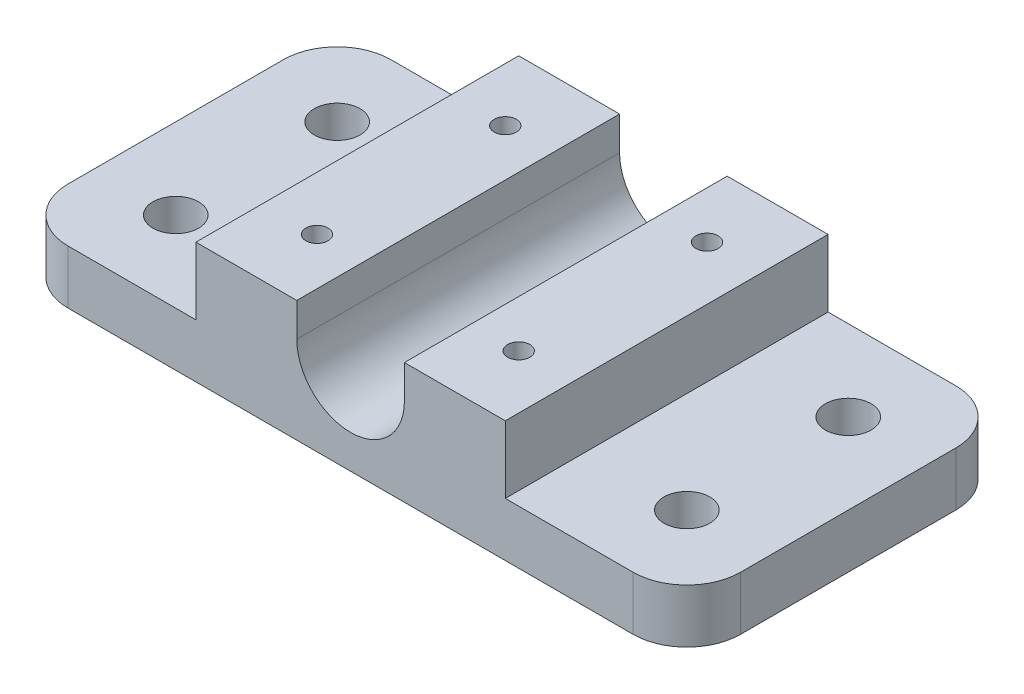
SolidWorks part; units mm, degrees
ref_plane "Front Plane" through (0, 0, 0) normal (0, 0, 1) x (1, 0, 0)
ref_plane "Top Plane" through (0, 0, 0) normal (0, 1, 0) x (1, 0, 0)
ref_plane "Right Plane" through (0, 0, 0) normal (1, 0, 0) x (0, 0, -1)
sketch "Sketch1" plane through (0, 0, 0) normal (0, 1, 0) x (1, 0, 0)
  line L1 (-50, 24) -> (50, 24)
  line L2 (-50, 24) -> (-50, -24)
  line L3 (-50, -24) -> (50, -24)
  line L4 (50, 24) -> (50, -24)
  line L5 (-50, 24) -> (50, -24) construction
  line L6 (-50, -24) -> (50, 24) construction
  point P0 (0, 0)
  dimension "D1" = 100
  dimension "D2" = 48
extrude "Boss-Extrude1" add sketch "Sketch1" along normal blind 8
sketch "Sketch2" plane through (0, 8, 0) normal (0, 1, 0) x (1, 0, 0)
  line L0 (-50, -24) -> (50, -24) construction
  line L1 (-23, 24) -> (23, 24)
  line L2 (-23, 24) -> (-23, -24)
  line L3 (-23, -24) -> (23, -24)
  line L4 (23, 24) -> (23, -24)
  line L5 (-23, 24) -> (23, -24) construction
  line L6 (-23, -24) -> (23, 24) construction
  point P0 (0, 0)
  dimension "D1" = 46
extrude "Boss-Extrude2" add sketch "Sketch2" along normal blind 10
sketch "Sketch3" plane through (0, 0, 24) normal (0, 0, 1) x (1, 0, 0)
  line L0 (0, 21) -> (0, 18) construction
  line L1 (-23, 18) -> (23, 18) construction
  line L3 (0, 13) -> (0, 18) construction
  line L4 (0, 5) -> (0, 18) construction
  line L5 (-8, 13) -> (-8, 18)
  line L6 (8, 13) -> (8, 18)
  line L7 (-8, 18) -> (8, 18)
  arc A0 (-8, 13) -> (8, 13) centre (0, 13) ccw
  dimension "D1" = 16
  dimension "D2" = 3
  dimension "D3" = 5
  dimension "D4" = 13
extrude "Cut-Extrude1" cut sketch "Sketch3" against normal through all
fillet "Fillet1" radius 8 4 edges at (50, 4, -24) (50, 4, 24) (-50, 4, -24) (-50, 4, 24)
hole_wizard "M4 Tapped Hole1" positions "Sketch5" profile "Sketch7" tap size "M4" standard "ISO"
sketch "Sketch5" plane through (0, 18, 0) normal (0, 1, 0) x (1, 0, 0)
  point P0 (-15, 14)
  point P3 (-15, -14)
  point P6 (15, -14)
  point P9 (15, 14)
sketch "Sketch7" plane through (-15, 18, -14) normal (1, 0, 0) x (0, 0, 1)
  line L0 (0, 0) -> (0, 10.9914)
  line L1 (0, 10.9914) -> (1.65, 10)
  line L2 (1.65, 10) -> (1.65, 0)
  line L5 (1.65, 0) -> (0, 0)
  line L10 (0, 10.9914) -> (-1.65, 10) construction
  line L11 (0, -6.35) -> (0, 107.95) construction
  dimension "Tap Drill Dia." = 3.3
  dimension "Tap Drill Depth" = 10
  dimension "Drill Angle" = 118
cosmetic thread "Hole Thread1" parameters "D1"=8, "D2"=4
cosmetic thread "Hole Thread2" parameters "D1"=8, "D2"=4
cosmetic thread "Hole Thread3" parameters "D1"=8, "D2"=4
cosmetic thread "Hole Thread4" parameters "D1"=8, "D2"=4
hole_wizard "M8 Tapped Hole1" positions "Sketch9" profile "Sketch11" tap size "M8" standard "ISO" end condition up to next
sketch "Sketch9" plane through (0, 8, 0) normal (0, 1, 0) x (1, 0, 0)
  line L0 (-38, 12) -> (38, 12) construction
  line L1 (38, 12) -> (38, -12) construction
  line L2 (38, -12) -> (-38, -12) construction
  line L3 (-38, -12) -> (-38, 12) construction
  line L5 (-50, 0) -> (50, 0) construction
  line L6 (-50, 16) -> (-50, -16) construction
  line L7 (50, -16) -> (50, 16) construction
  line L8 (8, 24) -> (-8, 24) construction
  point P0 (-38, 12)
  point P2 (-38, -12)
  point P4 (38, -12)
  point P6 (38, 12)
  point P25 (-38, 0)
  dimension "D1" = 76
  dimension "D2" = 12
  dimension "D3" = 12
  dimension "D4" = 24
  dimension "D5" = 12
  dimension "D6" = 12
sketch "Sketch11" plane through (-38, 8, -12) normal (1, 0, 0) x (0, 0, 1)
  line L0 (0, 0) -> (0, 8)
  line L1 (0, 8) -> (3.4, 8)
  line L2 (3.4, 8) -> (3.4, 0)
  line L5 (3.4, 0) -> (0, 0)
  line L11 (0, -6.35) -> (0, 107.95) construction
  dimension "Thru Tap Drill Dia." = 6.8
  dimension "Thru Tap Drill Depth" = 8
cosmetic thread "Hole Thread5" parameters "D2"=8
cosmetic thread "Hole Thread6" parameters "D2"=8
cosmetic thread "Hole Thread7" parameters "D2"=8
cosmetic thread "Hole Thread8" parameters "D2"=8
